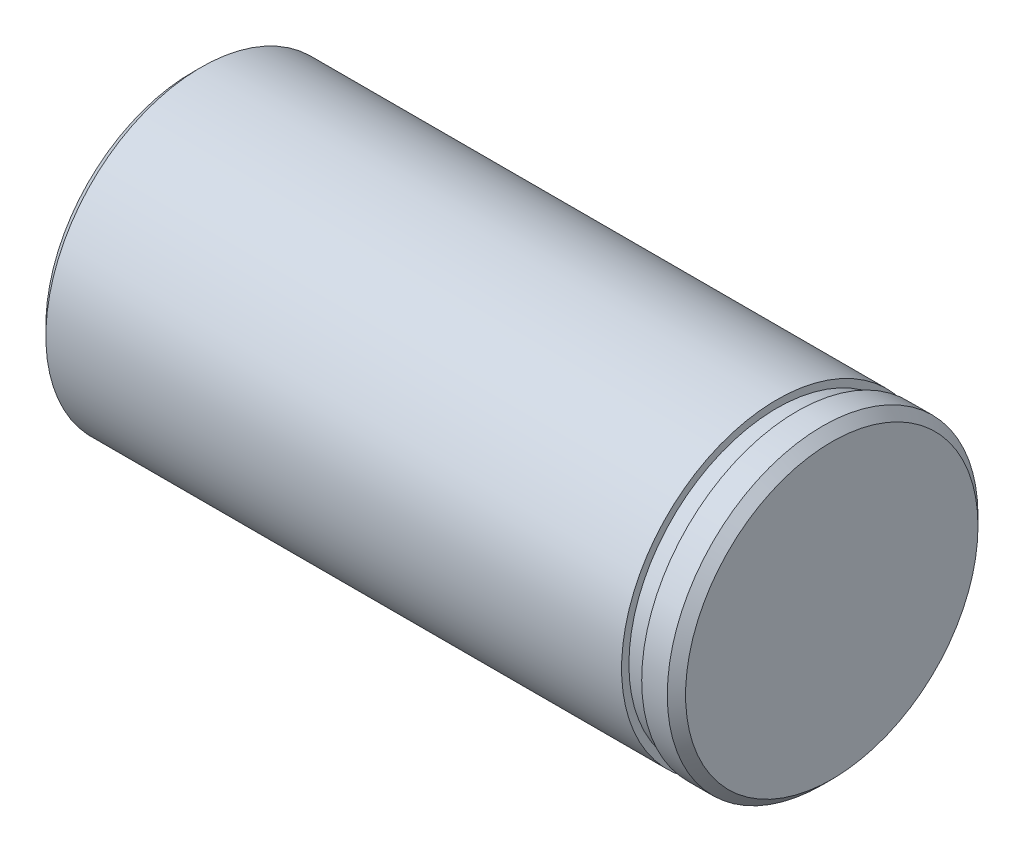
SolidWorks part; units mm, degrees
material "45"
ref_plane "前视基准面" through (0, 0, 0) normal (0, 0, 1) x (1, 0, 0)
ref_plane "上视基准面" through (0, 0, 0) normal (0, 1, 0) x (1, 0, 0)
ref_plane "右视基准面" through (0, 0, 0) normal (1, 0, 0) x (0, 0, -1)
sketch "草图1" plane through (0, 0, 0) normal (1, 0, 0) x (0, 0, -1)
  circle A0 centre (0, 0) radius 8.5
  dimension "D1" = 17
extrude "凸台-拉伸1" add sketch "草图1" along normal blind 35
hole_wizard "M6 螺纹孔1" positions "草图3" profile "草图2" tap size "M6" standard "ISO"
sketch "草图3" plane through (0, 0, 0) normal (-1, 0, 0) x (0, 0, 1)
  point P0 (0, 0)
sketch "草图2" plane through (0, 0, 0) normal (0, 1, 0) x (0, 0, 1)
  line L0 (0, 0) -> (0, 16.5022)
  line L1 (0, 16.5022) -> (2.5, 15)
  line L2 (2.5, 15) -> (2.5, 0)
  line L5 (2.5, 0) -> (0, 0)
  line L10 (0, 16.5022) -> (-2.5, 15) construction
  line L11 (0, -6.35) -> (0, 107.95) construction
  dimension "螺纹孔钻头直径" = 5
  dimension "螺纹孔钻头深度" = 15
  dimension "导头角度" = 118
cosmetic thread "孔螺蚊线1" parameters "D1"=12, "D2"=6
chamfer "倒角1" distance 0.5 angle 45 2 edges at (35, 0, -8.5) (0, 0, -8.5)
sketch "草图4" plane through (0, 0, 0) normal (0, 1, 0) x (1, 0, 0)
  line L0 (0, 8) -> (0, -8) construction
  line L1 (32, 10.8655) -> (33.1, 10.8655)
  line L2 (32, 10.8655) -> (32, 8.1)
  line L3 (32, 8.1) -> (33.1, 8.1)
  line L4 (33.1, 10.8655) -> (33.1, 8.1)
  line L5 (-5.2777, 0) -> (43.283, 0) construction
  dimension "D1" = 1.1
  dimension "D2" = 8.1
  dimension "D3" = 32
revolve "切除-旋转1" cut sketch "草图4" angle 360 about L5
